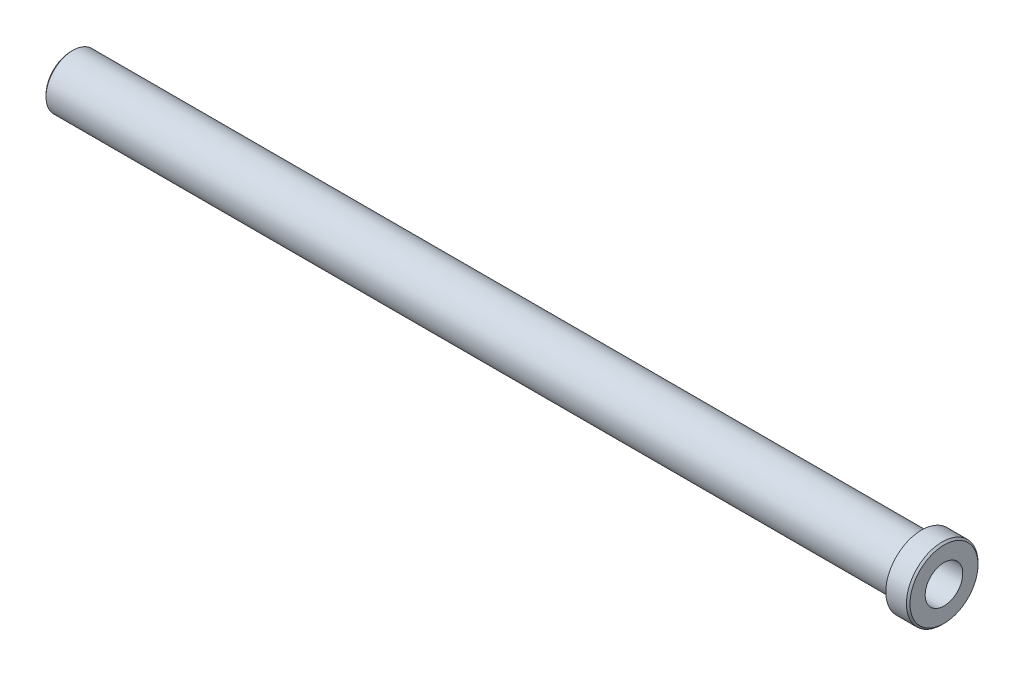
SolidWorks part; units mm, degrees
material "AISI 1045 钢，冷拔"
ref_plane "前视基准面" through (0, 0, 0) normal (0, 0, 1) x (1, 0, 0)
ref_plane "上视基准面" through (0, 0, 0) normal (0, 1, 0) x (1, 0, 0)
ref_plane "右视基准面" through (0, 0, 0) normal (1, 0, 0) x (0, 0, -1)
sketch "草图1" plane through (0, 0, 0) normal (1, 0, 0) x (0, 0, -1)
  circle A0 centre (0, 0) radius 30
extrude "凸台-拉伸1" add sketch "草图1" along normal mid plane 950 contours A0
sketch "草图2" plane through (475, 0, 0) normal (1, 0, 0) x (0, 0, -1)
  circle A0 centre (0, 0) radius 40
extrude "凸台-拉伸2" add sketch "草图2" along normal blind 25
chamfer "倒角1" distance 2 angle 45 1 edges at (500, 0, -40)
fillet "圆角1" radius 1 1 edges at (475, 0, -30)
sketch "草图3" plane through (-475, 0, 0) normal (-1, 0, 0) x (0, 0, 1)
  line L0 (0, 32.3037) -> (0, -33.3803) construction
  line L1 (-5.2, 23.673) -> (-5.2, 20.346)
  line L2 (5.2, 23.673) -> (5.2, 20.346)
  line L3 (5.2, 23.673) -> (5.2, 20.346)
  line L4 (13.0624, 20.4163) -> (10.7098, 18.0638)
  line L5 (20.4163, 13.0624) -> (18.0638, 10.7098)
  line L6 (23.673, 5.2) -> (20.346, 5.2)
  line L7 (23.673, -5.2) -> (20.346, -5.2)
  line L8 (20.4163, -13.0624) -> (18.0638, -10.7098)
  line L9 (13.0624, -20.4163) -> (10.7098, -18.0638)
  line L10 (5.2, -23.673) -> (5.2, -20.346)
  line L11 (-5.2, -23.673) -> (-5.2, -20.346)
  line L12 (-13.0624, -20.4163) -> (-10.7098, -18.0638)
  line L13 (-20.4163, -13.0624) -> (-18.0638, -10.7098)
  line L14 (-23.673, -5.2) -> (-20.346, -5.2)
  line L15 (-23.673, 5.2) -> (-20.346, 5.2)
  line L16 (-20.4163, 13.0624) -> (-18.0638, 10.7098)
  line L17 (-13.0624, 20.4163) -> (-10.7098, 18.0638)
  arc A0 (-5.2, 20.346) -> (-10.7098, 18.0638) centre (0, 0) ccw
  arc A1 (5.2, 23.673) -> (-5.2, 23.673) centre (0, 0) ccw
  arc A2 (20.4163, 13.0624) -> (13.0624, 20.4163) centre (0, 0) ccw
  arc A3 (23.673, -5.2) -> (23.673, 5.2) centre (0, 0) ccw
  arc A4 (13.0624, -20.4163) -> (20.4163, -13.0624) centre (0, 0) ccw
  arc A5 (-5.2, -23.673) -> (5.2, -23.673) centre (0, 0) ccw
  arc A6 (-20.4163, -13.0624) -> (-13.0624, -20.4163) centre (0, 0) ccw
  arc A7 (-23.673, 5.2) -> (-23.673, -5.2) centre (0, 0) ccw
  arc A8 (-13.0624, 20.4163) -> (-20.4163, 13.0624) centre (0, 0) ccw
  arc A9 (-18.0638, 10.7098) -> (-20.346, 5.2) centre (0, 0) ccw
  arc A10 (-20.346, -5.2) -> (-18.0638, -10.7098) centre (0, 0) ccw
  arc A11 (-10.7098, -18.0638) -> (-5.2, -20.346) centre (0, 0) ccw
  arc A12 (5.2, -20.346) -> (10.7098, -18.0638) centre (0, 0) ccw
  arc A13 (18.0638, -10.7098) -> (20.346, -5.2) centre (0, 0) ccw
  arc A14 (20.346, 5.2) -> (18.0638, 10.7098) centre (0, 0) ccw
  arc A15 (10.7098, 18.0638) -> (5.2, 20.346) centre (0, 0) ccw
  point P10 (5.2, 22.0095)
  point P40 (0, 0)
  dimension "D1" = 10.4
  dimension "D2" = 8
extrude "切除-拉伸2" cut sketch "草图3" against normal blind 120 contours L0 A1 L1 A0 L17 A8 L16 A9 L15 A7 L14 A10 L13 A6 L12 A11 L11 A5 | A1 L0 A5 L10 A12 L9 A4 L8 A13 L7 A3 L6 A14 L5 A2 L4 A15 L2
sketch "草图5" plane through (-355, 0, 0) normal (-1, 0, 0) x (0, 0, 1)
  circle A0 centre (0, 0) radius 21
extrude "切除-拉伸3" cut sketch "草图5" against normal through all
chamfer "倒角2" distance 2 angle 45 1 edges at (-475, 0, -30)
chamfer "倒角3" distance 1 angle 45 16 edges at (-475, -17.1384, -17.1384) (-475, -8.0364, -19.4015) (-475, -19.4015, -8.0364) (-475, -24.2374, 0) (-475, -19.4015, 8.0364) (-475, -17.1384, 17.1384) (-475, -8.0364, 19.4015) (-475, 0, 24.2374) (-475, 8.0364, 19.4015) (-475, 17.1384, 17.1384) (-475, 19.4015, 8.0364) (-475, 19.4015, -8.0364) (-475, 24.2374, 0) (-475, 17.1384, -17.1384) (-475, 0, -24.2374) (-475, 8.0364, -19.4015)
